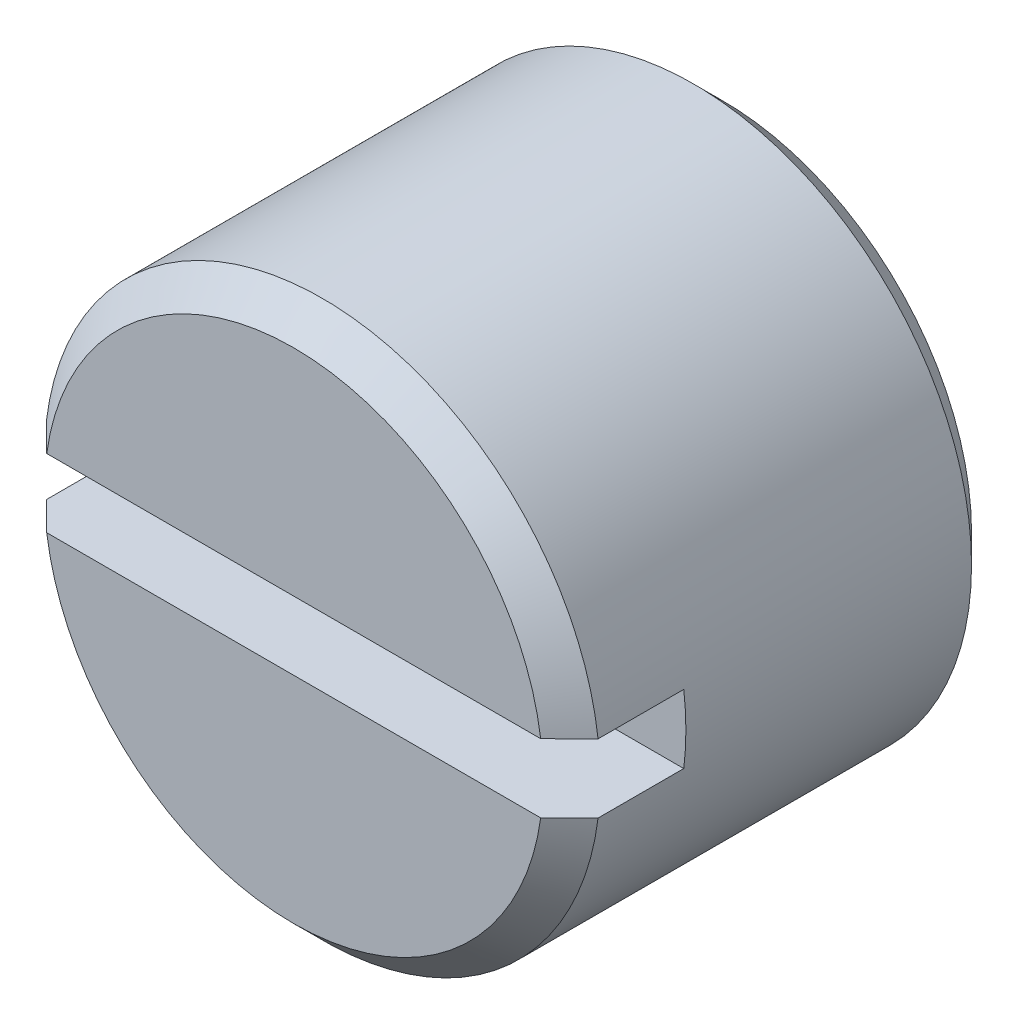
SolidWorks part; units mm, degrees
ref_plane "Front Plane" through (0, 0, 0) normal (0, 0, 1) x (1, 0, 0)
ref_plane "Top Plane" through (0, 0, 0) normal (0, 1, 0) x (1, 0, 0)
ref_plane "Right Plane" through (0, 0, 0) normal (1, 0, 0) x (0, 0, -1)
other "Configuration Table"
sketch "Sketch1" plane through (0, 0, 0) normal (0, 0, 1) x (1, 0, 0)
  circle A0 centre (0, 0) radius 4.865
  dimension "D1" = 9.73
extrude "Boss-Extrude1" add sketch "Sketch1" along normal blind 7.5
sketch "Sketch2" plane through (0, 0, 7.5) normal (0, 0, 1) x (1, 0, 0)
  line L1 (6.4102, -0.6) -> (-6.4102, -0.6)
  line L2 (6.4102, -0.6) -> (6.4102, 0.6)
  line L3 (6.4102, 0.6) -> (-6.4102, 0.6)
  line L4 (-6.4102, -0.6) -> (-6.4102, 0.6)
  line L5 (6.4102, -0.6) -> (-6.4102, 0.6) construction
  line L6 (6.4102, 0.6) -> (-6.4102, -0.6) construction
  point P0 (0, 0)
  dimension "D1" = 1.2
  dimension "D2" = 12.8203
extrude "Cut-Extrude1" cut sketch "Sketch2" against normal blind 2
chamfer "Chamfer1" distance 0.5 angle 45 3 edges at (4.865, 0, 0) (0, -4.865, 7.5) (0, 4.865, 7.5)
